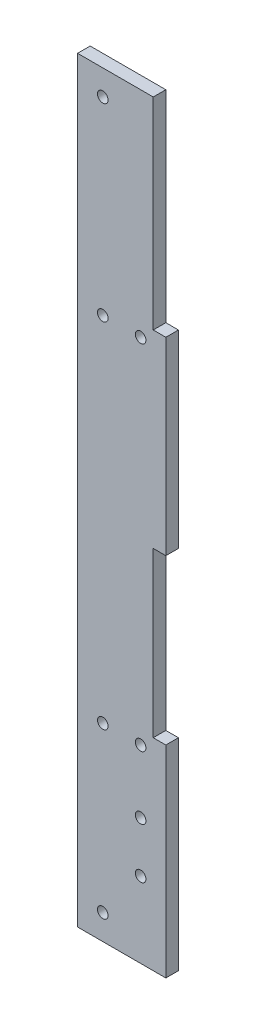
SolidWorks part; units mm, degrees
ref_plane "Front Plane" through (0, 0, 0) normal (0, 0, 1) x (1, 0, 0)
ref_plane "Top Plane" through (0, 0, 0) normal (0, 1, 0) x (1, 0, 0)
ref_plane "Right Plane" through (0, 0, 0) normal (1, 0, 0) x (0, 0, -1)
sketch "Sketch1" plane through (0, 0, 0) normal (0, 0, 1) x (1, 0, 0)
  line L0 (30, 300) -> (30, 220)
  line L1 (0, 0) -> (35, 0)
  line L2 (0, 0) -> (0, 300)
  line L3 (0, 300) -> (30, 300)
  line L4 (35, 0) -> (35, 80)
  line L5 (30, 220) -> (35, 220)
  line L6 (35, 145) -> (35, 220)
  line L7 (35, 145) -> (30, 145)
  line L8 (30, 145) -> (30, 80)
  line L9 (30, 80) -> (35, 80)
  circle A0 centre (25, 215) radius 2.1
  circle A1 centre (10, 215) radius 2.1
  circle A2 centre (25, 75) radius 2.1
  circle A3 centre (10, 75) radius 2.1
  circle A4 centre (10, 290) radius 2.1
  circle A5 centre (10, 10) radius 2.1
  circle A6 centre (25, 30) radius 2.1
  circle A7 centre (25, 50) radius 2.1
  point P15 (32.5, 220)
  dimension "D7" = 4.2
  dimension "D10" = 4.2
  dimension "D11" = 5
  dimension "D12" = 10
  dimension "D13" = 10
  dimension "D14" = 4.2
  dimension "D15" = 4.2
  dimension "D17" = 5
  dimension "D18" = 4.2
  dimension "D21" = 4.2
  dimension "D25" = 4.2
  dimension "D26" = 4.2
  dimension "D1" = 300
  dimension "D2" = 5
  dimension "D3" = 5
  dimension "D4" = 65
  dimension "D5" = 80
  dimension "D6" = 80
  dimension "D8" = 10
  dimension "D9" = 10
  dimension "D16" = 5
  dimension "D19" = 10
  dimension "D20" = 10
  dimension "D22" = 10
  dimension "D23" = 10
  dimension "D24" = 20
  dimension "D27" = 20
extrude "Boss-Extrude1" add sketch "Sketch1" along normal blind 5
